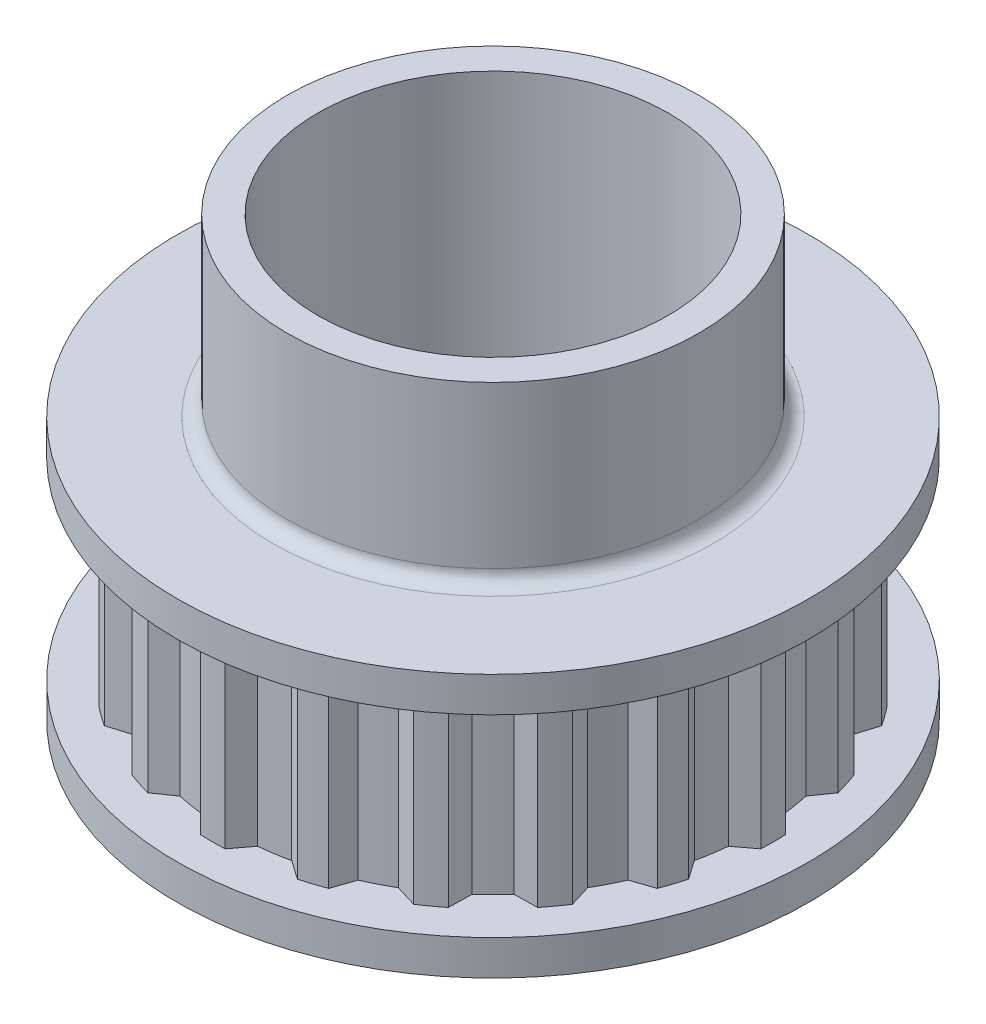
SolidWorks part; units mm, degrees
ref_plane "Front Plane" through (0, 0, 0) normal (0, 0, 1) x (1, 0, 0)
ref_plane "Top Plane" through (0, 0, 0) normal (0, 1, 0) x (1, 0, 0)
ref_plane "Right Plane" through (0, 0, 0) normal (1, 0, 0) x (0, 0, -1)
sketch "Sketch1" plane through (0, 0, 0) normal (0, 1, 0) x (1, 0, 0)
  circle A0 centre (0, 0) radius 16
  dimension "D1" = 32
extrude "Boss-Extrude1" add sketch "Sketch1" along normal blind 11
sketch "Sketch2" plane through (0, 11, 0) normal (0, 1, 0) x (1, 0, 0)
  line L0 (0, 21.2272) -> (0, -27.4763) construction
  line L1 (-1.5, 14.9329) -> (-0.7089, 15.9843)
  line L2 (1.5, 14.9329) -> (0.7089, 15.9843)
  line L3 (3.1879, 14.6656) -> (4.2652, 15.421)
  line L4 (6.0411, 13.7385) -> (5.6137, 14.9829)
  line L5 (7.5638, 12.9627) -> (8.8218, 13.3483)
  line L6 (9.9909, 11.1993) -> (9.9689, 12.5149)
  line L7 (11.1993, 9.9909) -> (12.5149, 9.9689)
  line L8 (12.9627, 7.5638) -> (13.3483, 8.8218)
  line L9 (13.7385, 6.0411) -> (14.9829, 5.6137)
  line L10 (14.6656, 3.1879) -> (15.421, 4.2652)
  line L11 (14.9329, 1.5) -> (15.9843, 0.7089)
  line L12 (14.9329, -1.5) -> (15.9843, -0.7089)
  line L13 (14.6656, -3.1879) -> (15.421, -4.2652)
  line L14 (13.7385, -6.0411) -> (14.9829, -5.6137)
  line L15 (12.9627, -7.5638) -> (13.3483, -8.8218)
  line L16 (11.1993, -9.9909) -> (12.5149, -9.9689)
  line L17 (9.9909, -11.1993) -> (9.9689, -12.5149)
  line L18 (7.5638, -12.9627) -> (8.8218, -13.3483)
  line L19 (6.0411, -13.7385) -> (5.6137, -14.9829)
  line L20 (3.1879, -14.6656) -> (4.2652, -15.421)
  line L21 (1.5, -14.9329) -> (0.7089, -15.9843)
  line L22 (-1.5, -14.9329) -> (-0.7089, -15.9843)
  line L23 (-3.1879, -14.6656) -> (-4.2652, -15.421)
  line L24 (-6.0411, -13.7385) -> (-5.6137, -14.9829)
  line L25 (-7.5638, -12.9627) -> (-8.8218, -13.3483)
  line L26 (-9.9909, -11.1993) -> (-9.9689, -12.5149)
  line L27 (-11.1993, -9.9909) -> (-12.5149, -9.9689)
  line L28 (-12.9627, -7.5638) -> (-13.3483, -8.8218)
  line L29 (-13.7385, -6.0411) -> (-14.9829, -5.6137)
  line L30 (-14.6656, -3.1879) -> (-15.421, -4.2652)
  line L31 (-14.9329, -1.5) -> (-15.9843, -0.7089)
  line L32 (-14.9329, 1.5) -> (-15.9843, 0.7089)
  line L33 (-14.6656, 3.1879) -> (-15.421, 4.2652)
  line L34 (-13.7385, 6.0411) -> (-14.9829, 5.6137)
  line L35 (-12.9627, 7.5638) -> (-13.3483, 8.8218)
  line L36 (-11.1993, 9.9909) -> (-12.5149, 9.9689)
  line L37 (-9.9909, 11.1993) -> (-9.9689, 12.5149)
  line L38 (-7.5638, 12.9627) -> (-8.8218, 13.3483)
  line L39 (-6.0411, 13.7385) -> (-5.6137, 14.9829)
  line L40 (-3.1879, 14.6656) -> (-4.2652, 15.421)
  arc A0 (-1.5, 14.9329) -> (-3.1879, 14.6656) centre (0, 0) ccw
  circle A1 centre (0, 0) radius 16 construction
  arc A3 (-1.5, 14.9329) -> (-3.1879, 14.6656) centre (0, 0) ccw
  arc A4 (5.6137, 14.9829) -> (4.2652, 15.421) centre (0, 0) ccw
  arc A5 (-1.5, 14.9329) -> (-3.1879, 14.6656) centre (0, 0) ccw
  arc A6 (9.9689, 12.5149) -> (8.8218, 13.3483) centre (0, 0) ccw
  arc A7 (-1.5, 14.9329) -> (-3.1879, 14.6656) centre (0, 0) ccw
  arc A8 (13.3483, 8.8218) -> (12.5149, 9.9689) centre (0, 0) ccw
  arc A9 (-1.5, 14.9329) -> (-3.1879, 14.6656) centre (0, 0) ccw
  arc A10 (15.9843, 0.7089) -> (15.421, 4.2652) centre (0, 0) ccw
  arc A11 (-1.5, 14.9329) -> (-3.1879, 14.6656) centre (0, 0) ccw
  arc A12 (15.421, -4.2652) -> (15.9843, -0.7089) centre (0, 0) ccw
  arc A13 (-1.5, 14.9329) -> (-3.1879, 14.6656) centre (0, 0) ccw
  arc A14 (13.3483, -8.8218) -> (14.9829, -5.6137) centre (0, 0) ccw
  arc A15 (-1.5, 14.9329) -> (-3.1879, 14.6656) centre (0, 0) ccw
  arc A16 (9.9689, -12.5149) -> (12.5149, -9.9689) centre (0, 0) ccw
  arc A17 (-1.5, 14.9329) -> (-3.1879, 14.6656) centre (0, 0) ccw
  arc A18 (5.6137, -14.9829) -> (8.8218, -13.3483) centre (0, 0) ccw
  arc A19 (-1.5, 14.9329) -> (-3.1879, 14.6656) centre (0, 0) ccw
  arc A20 (0.7089, -15.9843) -> (4.2652, -15.421) centre (0, 0) ccw
  arc A21 (-1.5, 14.9329) -> (-3.1879, 14.6656) centre (0, 0) ccw
  arc A22 (-4.2652, -15.421) -> (-0.7089, -15.9843) centre (0, 0) ccw
  arc A23 (-1.5, 14.9329) -> (-3.1879, 14.6656) centre (0, 0) ccw
  arc A24 (-8.8218, -13.3483) -> (-5.6137, -14.9829) centre (0, 0) ccw
  arc A25 (-1.5, 14.9329) -> (-3.1879, 14.6656) centre (0, 0) ccw
  arc A26 (-12.5149, -9.9689) -> (-9.9689, -12.5149) centre (0, 0) ccw
  arc A27 (-1.5, 14.9329) -> (-3.1879, 14.6656) centre (0, 0) ccw
  arc A28 (-14.9829, -5.6137) -> (-13.3483, -8.8218) centre (0, 0) ccw
  arc A29 (-1.5, 14.9329) -> (-3.1879, 14.6656) centre (0, 0) ccw
  arc A30 (-15.9843, -0.7089) -> (-15.421, -4.2652) centre (0, 0) ccw
  arc A31 (-1.5, 14.9329) -> (-3.1879, 14.6656) centre (0, 0) ccw
  arc A32 (-15.421, 4.2652) -> (-15.9843, 0.7089) centre (0, 0) ccw
  arc A33 (-1.5, 14.9329) -> (-3.1879, 14.6656) centre (0, 0) ccw
  arc A34 (-13.3483, 8.8218) -> (-14.9829, 5.6137) centre (0, 0) ccw
  arc A35 (-1.5, 14.9329) -> (-3.1879, 14.6656) centre (0, 0) ccw
  arc A36 (-9.9689, 12.5149) -> (-12.5149, 9.9689) centre (0, 0) ccw
  arc A37 (-1.5, 14.9329) -> (-3.1879, 14.6656) centre (0, 0) ccw
  arc A38 (-5.6137, 14.9829) -> (-8.8218, 13.3483) centre (0, 0) ccw
  arc A39 (-1.5, 14.9329) -> (-3.1879, 14.6656) centre (0, 0) ccw
  arc A40 (-0.7089, 15.9843) -> (-4.2652, 15.421) centre (0, 0) ccw
  arc A41 (3.1879, 14.6656) -> (1.5, 14.9329) centre (0, 0) ccw
  arc A42 (3.1879, 14.6656) -> (1.5, 14.9329) centre (0, 0) ccw
  arc A43 (3.1879, 14.6656) -> (1.5, 14.9329) centre (0, 0) ccw
  arc A44 (3.1879, 14.6656) -> (1.5, 14.9329) centre (0, 0) ccw
  arc A45 (3.1879, 14.6656) -> (1.5, 14.9329) centre (0, 0) ccw
  arc A46 (3.1879, 14.6656) -> (1.5, 14.9329) centre (0, 0) ccw
  arc A47 (3.1879, 14.6656) -> (1.5, 14.9329) centre (0, 0) ccw
  arc A48 (3.1879, 14.6656) -> (1.5, 14.9329) centre (0, 0) ccw
  arc A49 (3.1879, 14.6656) -> (1.5, 14.9329) centre (0, 0) ccw
  arc A50 (3.1879, 14.6656) -> (1.5, 14.9329) centre (0, 0) ccw
  arc A51 (3.1879, 14.6656) -> (1.5, 14.9329) centre (0, 0) ccw
  arc A52 (3.1879, 14.6656) -> (1.5, 14.9329) centre (0, 0) ccw
  arc A53 (3.1879, 14.6656) -> (1.5, 14.9329) centre (0, 0) ccw
  arc A54 (3.1879, 14.6656) -> (1.5, 14.9329) centre (0, 0) ccw
  arc A55 (3.1879, 14.6656) -> (1.5, 14.9329) centre (0, 0) ccw
  arc A56 (3.1879, 14.6656) -> (1.5, 14.9329) centre (0, 0) ccw
  arc A57 (3.1879, 14.6656) -> (1.5, 14.9329) centre (0, 0) ccw
  arc A58 (3.1879, 14.6656) -> (1.5, 14.9329) centre (0, 0) ccw
  arc A59 (3.1879, 14.6656) -> (1.5, 14.9329) centre (0, 0) ccw
  arc A60 (3.1879, 14.6656) -> (1.5, 14.9329) centre (0, 0) ccw
  arc A61 (7.5638, 12.9627) -> (6.0411, 13.7385) centre (0, 0) ccw
  arc A62 (7.5638, 12.9627) -> (6.0411, 13.7385) centre (0, 0) ccw
  arc A63 (7.5638, 12.9627) -> (6.0411, 13.7385) centre (0, 0) ccw
  arc A64 (7.5638, 12.9627) -> (6.0411, 13.7385) centre (0, 0) ccw
  arc A65 (7.5638, 12.9627) -> (6.0411, 13.7385) centre (0, 0) ccw
  arc A66 (7.5638, 12.9627) -> (6.0411, 13.7385) centre (0, 0) ccw
  arc A67 (7.5638, 12.9627) -> (6.0411, 13.7385) centre (0, 0) ccw
  arc A68 (7.5638, 12.9627) -> (6.0411, 13.7385) centre (0, 0) ccw
  arc A69 (7.5638, 12.9627) -> (6.0411, 13.7385) centre (0, 0) ccw
  arc A70 (7.5638, 12.9627) -> (6.0411, 13.7385) centre (0, 0) ccw
  arc A71 (7.5638, 12.9627) -> (6.0411, 13.7385) centre (0, 0) ccw
  arc A72 (7.5638, 12.9627) -> (6.0411, 13.7385) centre (0, 0) ccw
  arc A73 (7.5638, 12.9627) -> (6.0411, 13.7385) centre (0, 0) ccw
  arc A74 (7.5638, 12.9627) -> (6.0411, 13.7385) centre (0, 0) ccw
  arc A75 (7.5638, 12.9627) -> (6.0411, 13.7385) centre (0, 0) ccw
  arc A76 (7.5638, 12.9627) -> (6.0411, 13.7385) centre (0, 0) ccw
  arc A77 (7.5638, 12.9627) -> (6.0411, 13.7385) centre (0, 0) ccw
  arc A78 (7.5638, 12.9627) -> (6.0411, 13.7385) centre (0, 0) ccw
  arc A79 (7.5638, 12.9627) -> (6.0411, 13.7385) centre (0, 0) ccw
  arc A80 (7.5638, 12.9627) -> (6.0411, 13.7385) centre (0, 0) ccw
  arc A81 (11.1993, 9.9909) -> (9.9909, 11.1993) centre (0, 0) ccw
  arc A82 (11.1993, 9.9909) -> (9.9909, 11.1993) centre (0, 0) ccw
  arc A83 (11.1993, 9.9909) -> (9.9909, 11.1993) centre (0, 0) ccw
  arc A84 (11.1993, 9.9909) -> (9.9909, 11.1993) centre (0, 0) ccw
  arc A85 (11.1993, 9.9909) -> (9.9909, 11.1993) centre (0, 0) ccw
  arc A86 (11.1993, 9.9909) -> (9.9909, 11.1993) centre (0, 0) ccw
  arc A87 (11.1993, 9.9909) -> (9.9909, 11.1993) centre (0, 0) ccw
  arc A88 (11.1993, 9.9909) -> (9.9909, 11.1993) centre (0, 0) ccw
  arc A89 (11.1993, 9.9909) -> (9.9909, 11.1993) centre (0, 0) ccw
  arc A90 (11.1993, 9.9909) -> (9.9909, 11.1993) centre (0, 0) ccw
  arc A91 (11.1993, 9.9909) -> (9.9909, 11.1993) centre (0, 0) ccw
  arc A92 (11.1993, 9.9909) -> (9.9909, 11.1993) centre (0, 0) ccw
  arc A93 (11.1993, 9.9909) -> (9.9909, 11.1993) centre (0, 0) ccw
  arc A94 (11.1993, 9.9909) -> (9.9909, 11.1993) centre (0, 0) ccw
  arc A95 (11.1993, 9.9909) -> (9.9909, 11.1993) centre (0, 0) ccw
  arc A96 (11.1993, 9.9909) -> (9.9909, 11.1993) centre (0, 0) ccw
  arc A97 (11.1993, 9.9909) -> (9.9909, 11.1993) centre (0, 0) ccw
  arc A98 (11.1993, 9.9909) -> (9.9909, 11.1993) centre (0, 0) ccw
  arc A99 (11.1993, 9.9909) -> (9.9909, 11.1993) centre (0, 0) ccw
  arc A100 (11.1993, 9.9909) -> (9.9909, 11.1993) centre (0, 0) ccw
  arc A101 (13.7385, 6.0411) -> (12.9627, 7.5638) centre (0, 0) ccw
  arc A102 (13.7385, 6.0411) -> (12.9627, 7.5638) centre (0, 0) ccw
  arc A103 (13.7385, 6.0411) -> (12.9627, 7.5638) centre (0, 0) ccw
  arc A104 (13.7385, 6.0411) -> (12.9627, 7.5638) centre (0, 0) ccw
  arc A105 (13.7385, 6.0411) -> (12.9627, 7.5638) centre (0, 0) ccw
  arc A106 (13.7385, 6.0411) -> (12.9627, 7.5638) centre (0, 0) ccw
  arc A107 (13.7385, 6.0411) -> (12.9627, 7.5638) centre (0, 0) ccw
  arc A108 (13.7385, 6.0411) -> (12.9627, 7.5638) centre (0, 0) ccw
  arc A109 (13.7385, 6.0411) -> (12.9627, 7.5638) centre (0, 0) ccw
  arc A110 (13.7385, 6.0411) -> (12.9627, 7.5638) centre (0, 0) ccw
  arc A111 (13.7385, 6.0411) -> (12.9627, 7.5638) centre (0, 0) ccw
  arc A112 (13.7385, 6.0411) -> (12.9627, 7.5638) centre (0, 0) ccw
  arc A113 (13.7385, 6.0411) -> (12.9627, 7.5638) centre (0, 0) ccw
  arc A114 (13.7385, 6.0411) -> (12.9627, 7.5638) centre (0, 0) ccw
  arc A115 (13.7385, 6.0411) -> (12.9627, 7.5638) centre (0, 0) ccw
  arc A116 (13.7385, 6.0411) -> (12.9627, 7.5638) centre (0, 0) ccw
  arc A117 (13.7385, 6.0411) -> (12.9627, 7.5638) centre (0, 0) ccw
  arc A118 (13.7385, 6.0411) -> (12.9627, 7.5638) centre (0, 0) ccw
  arc A119 (13.7385, 6.0411) -> (12.9627, 7.5638) centre (0, 0) ccw
  arc A120 (13.7385, 6.0411) -> (12.9627, 7.5638) centre (0, 0) ccw
  arc A121 (14.9329, 1.5) -> (14.6656, 3.1879) centre (0, 0) ccw
  arc A122 (14.9329, 1.5) -> (14.6656, 3.1879) centre (0, 0) ccw
  arc A123 (14.9329, 1.5) -> (14.6656, 3.1879) centre (0, 0) ccw
  arc A124 (14.9329, 1.5) -> (14.6656, 3.1879) centre (0, 0) ccw
  arc A125 (14.9329, 1.5) -> (14.6656, 3.1879) centre (0, 0) ccw
  arc A126 (14.9329, 1.5) -> (14.6656, 3.1879) centre (0, 0) ccw
  arc A127 (14.9329, 1.5) -> (14.6656, 3.1879) centre (0, 0) ccw
  arc A128 (14.9329, 1.5) -> (14.6656, 3.1879) centre (0, 0) ccw
  arc A129 (14.9329, 1.5) -> (14.6656, 3.1879) centre (0, 0) ccw
  arc A130 (14.9329, 1.5) -> (14.6656, 3.1879) centre (0, 0) ccw
  arc A131 (14.9329, 1.5) -> (14.6656, 3.1879) centre (0, 0) ccw
  arc A132 (14.9329, 1.5) -> (14.6656, 3.1879) centre (0, 0) ccw
  arc A133 (14.9329, 1.5) -> (14.6656, 3.1879) centre (0, 0) ccw
  arc A134 (14.9329, 1.5) -> (14.6656, 3.1879) centre (0, 0) ccw
  arc A135 (14.9329, 1.5) -> (14.6656, 3.1879) centre (0, 0) ccw
  arc A136 (14.9329, 1.5) -> (14.6656, 3.1879) centre (0, 0) ccw
  arc A137 (14.9329, 1.5) -> (14.6656, 3.1879) centre (0, 0) ccw
  arc A138 (14.9329, 1.5) -> (14.6656, 3.1879) centre (0, 0) ccw
  arc A139 (14.9329, 1.5) -> (14.6656, 3.1879) centre (0, 0) ccw
  arc A140 (14.9329, 1.5) -> (14.6656, 3.1879) centre (0, 0) ccw
  arc A141 (14.6656, -3.1879) -> (14.9329, -1.5) centre (0, 0) ccw
  arc A142 (14.6656, -3.1879) -> (14.9329, -1.5) centre (0, 0) ccw
  arc A143 (14.6656, -3.1879) -> (14.9329, -1.5) centre (0, 0) ccw
  arc A144 (14.6656, -3.1879) -> (14.9329, -1.5) centre (0, 0) ccw
  arc A145 (14.6656, -3.1879) -> (14.9329, -1.5) centre (0, 0) ccw
  arc A146 (14.6656, -3.1879) -> (14.9329, -1.5) centre (0, 0) ccw
  arc A147 (14.6656, -3.1879) -> (14.9329, -1.5) centre (0, 0) ccw
  arc A148 (14.6656, -3.1879) -> (14.9329, -1.5) centre (0, 0) ccw
  arc A149 (14.6656, -3.1879) -> (14.9329, -1.5) centre (0, 0) ccw
  arc A150 (14.6656, -3.1879) -> (14.9329, -1.5) centre (0, 0) ccw
  arc A151 (14.6656, -3.1879) -> (14.9329, -1.5) centre (0, 0) ccw
  arc A152 (14.6656, -3.1879) -> (14.9329, -1.5) centre (0, 0) ccw
  arc A153 (14.6656, -3.1879) -> (14.9329, -1.5) centre (0, 0) ccw
  arc A154 (14.6656, -3.1879) -> (14.9329, -1.5) centre (0, 0) ccw
  arc A155 (14.6656, -3.1879) -> (14.9329, -1.5) centre (0, 0) ccw
  arc A156 (14.6656, -3.1879) -> (14.9329, -1.5) centre (0, 0) ccw
  arc A157 (14.6656, -3.1879) -> (14.9329, -1.5) centre (0, 0) ccw
  arc A158 (14.6656, -3.1879) -> (14.9329, -1.5) centre (0, 0) ccw
  arc A159 (14.6656, -3.1879) -> (14.9329, -1.5) centre (0, 0) ccw
  arc A160 (14.6656, -3.1879) -> (14.9329, -1.5) centre (0, 0) ccw
  arc A161 (12.9627, -7.5638) -> (13.7385, -6.0411) centre (0, 0) ccw
  arc A162 (12.9627, -7.5638) -> (13.7385, -6.0411) centre (0, 0) ccw
  arc A163 (12.9627, -7.5638) -> (13.7385, -6.0411) centre (0, 0) ccw
  arc A164 (12.9627, -7.5638) -> (13.7385, -6.0411) centre (0, 0) ccw
  arc A165 (12.9627, -7.5638) -> (13.7385, -6.0411) centre (0, 0) ccw
  arc A166 (12.9627, -7.5638) -> (13.7385, -6.0411) centre (0, 0) ccw
  arc A167 (12.9627, -7.5638) -> (13.7385, -6.0411) centre (0, 0) ccw
  arc A168 (12.9627, -7.5638) -> (13.7385, -6.0411) centre (0, 0) ccw
  arc A169 (12.9627, -7.5638) -> (13.7385, -6.0411) centre (0, 0) ccw
  arc A170 (12.9627, -7.5638) -> (13.7385, -6.0411) centre (0, 0) ccw
  arc A171 (12.9627, -7.5638) -> (13.7385, -6.0411) centre (0, 0) ccw
  arc A172 (12.9627, -7.5638) -> (13.7385, -6.0411) centre (0, 0) ccw
  arc A173 (12.9627, -7.5638) -> (13.7385, -6.0411) centre (0, 0) ccw
  arc A174 (12.9627, -7.5638) -> (13.7385, -6.0411) centre (0, 0) ccw
  arc A175 (12.9627, -7.5638) -> (13.7385, -6.0411) centre (0, 0) ccw
  arc A176 (12.9627, -7.5638) -> (13.7385, -6.0411) centre (0, 0) ccw
  arc A177 (12.9627, -7.5638) -> (13.7385, -6.0411) centre (0, 0) ccw
  arc A178 (12.9627, -7.5638) -> (13.7385, -6.0411) centre (0, 0) ccw
  arc A179 (12.9627, -7.5638) -> (13.7385, -6.0411) centre (0, 0) ccw
  arc A180 (12.9627, -7.5638) -> (13.7385, -6.0411) centre (0, 0) ccw
  arc A181 (9.9909, -11.1993) -> (11.1993, -9.9909) centre (0, 0) ccw
  arc A182 (9.9909, -11.1993) -> (11.1993, -9.9909) centre (0, 0) ccw
  arc A183 (9.9909, -11.1993) -> (11.1993, -9.9909) centre (0, 0) ccw
  arc A184 (9.9909, -11.1993) -> (11.1993, -9.9909) centre (0, 0) ccw
  arc A185 (9.9909, -11.1993) -> (11.1993, -9.9909) centre (0, 0) ccw
  arc A186 (9.9909, -11.1993) -> (11.1993, -9.9909) centre (0, 0) ccw
  arc A187 (9.9909, -11.1993) -> (11.1993, -9.9909) centre (0, 0) ccw
  arc A188 (9.9909, -11.1993) -> (11.1993, -9.9909) centre (0, 0) ccw
  arc A189 (9.9909, -11.1993) -> (11.1993, -9.9909) centre (0, 0) ccw
  arc A190 (9.9909, -11.1993) -> (11.1993, -9.9909) centre (0, 0) ccw
  arc A191 (9.9909, -11.1993) -> (11.1993, -9.9909) centre (0, 0) ccw
  arc A192 (9.9909, -11.1993) -> (11.1993, -9.9909) centre (0, 0) ccw
  arc A193 (9.9909, -11.1993) -> (11.1993, -9.9909) centre (0, 0) ccw
  arc A194 (9.9909, -11.1993) -> (11.1993, -9.9909) centre (0, 0) ccw
  arc A195 (9.9909, -11.1993) -> (11.1993, -9.9909) centre (0, 0) ccw
  arc A196 (9.9909, -11.1993) -> (11.1993, -9.9909) centre (0, 0) ccw
  arc A197 (9.9909, -11.1993) -> (11.1993, -9.9909) centre (0, 0) ccw
  arc A198 (9.9909, -11.1993) -> (11.1993, -9.9909) centre (0, 0) ccw
  arc A199 (9.9909, -11.1993) -> (11.1993, -9.9909) centre (0, 0) ccw
  arc A200 (9.9909, -11.1993) -> (11.1993, -9.9909) centre (0, 0) ccw
  arc A201 (1.5, -14.9329) -> (3.1879, -14.6656) centre (0, 0) ccw
  arc A202 (1.5, -14.9329) -> (3.1879, -14.6656) centre (0, 0) ccw
  arc A203 (1.5, -14.9329) -> (3.1879, -14.6656) centre (0, 0) ccw
  arc A204 (1.5, -14.9329) -> (3.1879, -14.6656) centre (0, 0) ccw
  arc A205 (1.5, -14.9329) -> (3.1879, -14.6656) centre (0, 0) ccw
  arc A206 (1.5, -14.9329) -> (3.1879, -14.6656) centre (0, 0) ccw
  arc A207 (1.5, -14.9329) -> (3.1879, -14.6656) centre (0, 0) ccw
  arc A208 (1.5, -14.9329) -> (3.1879, -14.6656) centre (0, 0) ccw
  arc A209 (1.5, -14.9329) -> (3.1879, -14.6656) centre (0, 0) ccw
  arc A210 (1.5, -14.9329) -> (3.1879, -14.6656) centre (0, 0) ccw
  arc A211 (1.5, -14.9329) -> (3.1879, -14.6656) centre (0, 0) ccw
  arc A212 (1.5, -14.9329) -> (3.1879, -14.6656) centre (0, 0) ccw
  arc A213 (1.5, -14.9329) -> (3.1879, -14.6656) centre (0, 0) ccw
  arc A214 (1.5, -14.9329) -> (3.1879, -14.6656) centre (0, 0) ccw
  arc A215 (1.5, -14.9329) -> (3.1879, -14.6656) centre (0, 0) ccw
  arc A216 (1.5, -14.9329) -> (3.1879, -14.6656) centre (0, 0) ccw
  arc A217 (1.5, -14.9329) -> (3.1879, -14.6656) centre (0, 0) ccw
  arc A218 (1.5, -14.9329) -> (3.1879, -14.6656) centre (0, 0) ccw
  arc A219 (1.5, -14.9329) -> (3.1879, -14.6656) centre (0, 0) ccw
  arc A220 (1.5, -14.9329) -> (3.1879, -14.6656) centre (0, 0) ccw
  arc A221 (-3.1879, -14.6656) -> (-1.5, -14.9329) centre (0, 0) ccw
  arc A222 (-3.1879, -14.6656) -> (-1.5, -14.9329) centre (0, 0) ccw
  arc A223 (-3.1879, -14.6656) -> (-1.5, -14.9329) centre (0, 0) ccw
  arc A224 (-3.1879, -14.6656) -> (-1.5, -14.9329) centre (0, 0) ccw
  arc A225 (-3.1879, -14.6656) -> (-1.5, -14.9329) centre (0, 0) ccw
  arc A226 (-3.1879, -14.6656) -> (-1.5, -14.9329) centre (0, 0) ccw
  arc A227 (-3.1879, -14.6656) -> (-1.5, -14.9329) centre (0, 0) ccw
  arc A228 (-3.1879, -14.6656) -> (-1.5, -14.9329) centre (0, 0) ccw
  arc A229 (-3.1879, -14.6656) -> (-1.5, -14.9329) centre (0, 0) ccw
  arc A230 (-3.1879, -14.6656) -> (-1.5, -14.9329) centre (0, 0) ccw
  arc A231 (-3.1879, -14.6656) -> (-1.5, -14.9329) centre (0, 0) ccw
  arc A232 (-3.1879, -14.6656) -> (-1.5, -14.9329) centre (0, 0) ccw
  arc A233 (-3.1879, -14.6656) -> (-1.5, -14.9329) centre (0, 0) ccw
  arc A234 (-3.1879, -14.6656) -> (-1.5, -14.9329) centre (0, 0) ccw
  arc A235 (-3.1879, -14.6656) -> (-1.5, -14.9329) centre (0, 0) ccw
  arc A236 (-3.1879, -14.6656) -> (-1.5, -14.9329) centre (0, 0) ccw
  arc A237 (-3.1879, -14.6656) -> (-1.5, -14.9329) centre (0, 0) ccw
  arc A238 (-3.1879, -14.6656) -> (-1.5, -14.9329) centre (0, 0) ccw
  arc A239 (-3.1879, -14.6656) -> (-1.5, -14.9329) centre (0, 0) ccw
  arc A240 (-3.1879, -14.6656) -> (-1.5, -14.9329) centre (0, 0) ccw
  arc A241 (-7.5638, -12.9627) -> (-6.0411, -13.7385) centre (0, 0) ccw
  arc A242 (-7.5638, -12.9627) -> (-6.0411, -13.7385) centre (0, 0) ccw
  arc A243 (-7.5638, -12.9627) -> (-6.0411, -13.7385) centre (0, 0) ccw
  arc A244 (-7.5638, -12.9627) -> (-6.0411, -13.7385) centre (0, 0) ccw
  arc A245 (-7.5638, -12.9627) -> (-6.0411, -13.7385) centre (0, 0) ccw
  arc A246 (-7.5638, -12.9627) -> (-6.0411, -13.7385) centre (0, 0) ccw
  arc A247 (-7.5638, -12.9627) -> (-6.0411, -13.7385) centre (0, 0) ccw
  arc A248 (-7.5638, -12.9627) -> (-6.0411, -13.7385) centre (0, 0) ccw
  arc A249 (-7.5638, -12.9627) -> (-6.0411, -13.7385) centre (0, 0) ccw
  arc A250 (-7.5638, -12.9627) -> (-6.0411, -13.7385) centre (0, 0) ccw
  arc A251 (-7.5638, -12.9627) -> (-6.0411, -13.7385) centre (0, 0) ccw
  arc A252 (-7.5638, -12.9627) -> (-6.0411, -13.7385) centre (0, 0) ccw
  arc A253 (-7.5638, -12.9627) -> (-6.0411, -13.7385) centre (0, 0) ccw
  arc A254 (-7.5638, -12.9627) -> (-6.0411, -13.7385) centre (0, 0) ccw
  arc A255 (-7.5638, -12.9627) -> (-6.0411, -13.7385) centre (0, 0) ccw
  arc A256 (-7.5638, -12.9627) -> (-6.0411, -13.7385) centre (0, 0) ccw
  arc A257 (-7.5638, -12.9627) -> (-6.0411, -13.7385) centre (0, 0) ccw
  arc A258 (-7.5638, -12.9627) -> (-6.0411, -13.7385) centre (0, 0) ccw
  arc A259 (-7.5638, -12.9627) -> (-6.0411, -13.7385) centre (0, 0) ccw
  arc A260 (-7.5638, -12.9627) -> (-6.0411, -13.7385) centre (0, 0) ccw
  arc A261 (-11.1993, -9.9909) -> (-9.9909, -11.1993) centre (0, 0) ccw
  arc A262 (-11.1993, -9.9909) -> (-9.9909, -11.1993) centre (0, 0) ccw
  arc A263 (-11.1993, -9.9909) -> (-9.9909, -11.1993) centre (0, 0) ccw
  arc A264 (-11.1993, -9.9909) -> (-9.9909, -11.1993) centre (0, 0) ccw
  arc A265 (-11.1993, -9.9909) -> (-9.9909, -11.1993) centre (0, 0) ccw
  arc A266 (-11.1993, -9.9909) -> (-9.9909, -11.1993) centre (0, 0) ccw
  arc A267 (-11.1993, -9.9909) -> (-9.9909, -11.1993) centre (0, 0) ccw
  arc A268 (-11.1993, -9.9909) -> (-9.9909, -11.1993) centre (0, 0) ccw
  arc A269 (-11.1993, -9.9909) -> (-9.9909, -11.1993) centre (0, 0) ccw
  arc A270 (-11.1993, -9.9909) -> (-9.9909, -11.1993) centre (0, 0) ccw
  arc A271 (-11.1993, -9.9909) -> (-9.9909, -11.1993) centre (0, 0) ccw
  arc A272 (-11.1993, -9.9909) -> (-9.9909, -11.1993) centre (0, 0) ccw
  arc A273 (-11.1993, -9.9909) -> (-9.9909, -11.1993) centre (0, 0) ccw
  arc A274 (-11.1993, -9.9909) -> (-9.9909, -11.1993) centre (0, 0) ccw
  arc A275 (-11.1993, -9.9909) -> (-9.9909, -11.1993) centre (0, 0) ccw
  arc A276 (-11.1993, -9.9909) -> (-9.9909, -11.1993) centre (0, 0) ccw
  arc A277 (-11.1993, -9.9909) -> (-9.9909, -11.1993) centre (0, 0) ccw
  arc A278 (-11.1993, -9.9909) -> (-9.9909, -11.1993) centre (0, 0) ccw
  arc A279 (-11.1993, -9.9909) -> (-9.9909, -11.1993) centre (0, 0) ccw
  arc A280 (-11.1993, -9.9909) -> (-9.9909, -11.1993) centre (0, 0) ccw
  arc A281 (-13.7385, -6.0411) -> (-12.9627, -7.5638) centre (0, 0) ccw
  arc A282 (-13.7385, -6.0411) -> (-12.9627, -7.5638) centre (0, 0) ccw
  arc A283 (-13.7385, -6.0411) -> (-12.9627, -7.5638) centre (0, 0) ccw
  arc A284 (-13.7385, -6.0411) -> (-12.9627, -7.5638) centre (0, 0) ccw
  arc A285 (-13.7385, -6.0411) -> (-12.9627, -7.5638) centre (0, 0) ccw
  arc A286 (-13.7385, -6.0411) -> (-12.9627, -7.5638) centre (0, 0) ccw
  arc A287 (-13.7385, -6.0411) -> (-12.9627, -7.5638) centre (0, 0) ccw
  arc A288 (-13.7385, -6.0411) -> (-12.9627, -7.5638) centre (0, 0) ccw
  arc A289 (-13.7385, -6.0411) -> (-12.9627, -7.5638) centre (0, 0) ccw
  arc A290 (-13.7385, -6.0411) -> (-12.9627, -7.5638) centre (0, 0) ccw
  arc A291 (-13.7385, -6.0411) -> (-12.9627, -7.5638) centre (0, 0) ccw
  arc A292 (-13.7385, -6.0411) -> (-12.9627, -7.5638) centre (0, 0) ccw
  arc A293 (-13.7385, -6.0411) -> (-12.9627, -7.5638) centre (0, 0) ccw
  arc A294 (-13.7385, -6.0411) -> (-12.9627, -7.5638) centre (0, 0) ccw
  arc A295 (-13.7385, -6.0411) -> (-12.9627, -7.5638) centre (0, 0) ccw
  arc A296 (-13.7385, -6.0411) -> (-12.9627, -7.5638) centre (0, 0) ccw
  arc A297 (-13.7385, -6.0411) -> (-12.9627, -7.5638) centre (0, 0) ccw
  arc A298 (-13.7385, -6.0411) -> (-12.9627, -7.5638) centre (0, 0) ccw
  arc A299 (-13.7385, -6.0411) -> (-12.9627, -7.5638) centre (0, 0) ccw
  arc A300 (-13.7385, -6.0411) -> (-12.9627, -7.5638) centre (0, 0) ccw
  arc A301 (-14.9329, -1.5) -> (-14.6656, -3.1879) centre (0, 0) ccw
  arc A302 (-14.9329, -1.5) -> (-14.6656, -3.1879) centre (0, 0) ccw
  arc A303 (-14.9329, -1.5) -> (-14.6656, -3.1879) centre (0, 0) ccw
  arc A304 (-14.9329, -1.5) -> (-14.6656, -3.1879) centre (0, 0) ccw
  arc A305 (-14.9329, -1.5) -> (-14.6656, -3.1879) centre (0, 0) ccw
  arc A306 (-14.9329, -1.5) -> (-14.6656, -3.1879) centre (0, 0) ccw
  arc A307 (-14.9329, -1.5) -> (-14.6656, -3.1879) centre (0, 0) ccw
  arc A308 (-14.9329, -1.5) -> (-14.6656, -3.1879) centre (0, 0) ccw
  arc A309 (-14.9329, -1.5) -> (-14.6656, -3.1879) centre (0, 0) ccw
  arc A310 (-14.9329, -1.5) -> (-14.6656, -3.1879) centre (0, 0) ccw
  arc A311 (-14.9329, -1.5) -> (-14.6656, -3.1879) centre (0, 0) ccw
  arc A312 (-14.9329, -1.5) -> (-14.6656, -3.1879) centre (0, 0) ccw
  arc A313 (-14.9329, -1.5) -> (-14.6656, -3.1879) centre (0, 0) ccw
  arc A314 (-14.9329, -1.5) -> (-14.6656, -3.1879) centre (0, 0) ccw
  arc A315 (-14.9329, -1.5) -> (-14.6656, -3.1879) centre (0, 0) ccw
  arc A316 (-14.9329, -1.5) -> (-14.6656, -3.1879) centre (0, 0) ccw
  arc A317 (-14.9329, -1.5) -> (-14.6656, -3.1879) centre (0, 0) ccw
  arc A318 (-14.9329, -1.5) -> (-14.6656, -3.1879) centre (0, 0) ccw
  arc A319 (-14.9329, -1.5) -> (-14.6656, -3.1879) centre (0, 0) ccw
  arc A320 (-14.9329, -1.5) -> (-14.6656, -3.1879) centre (0, 0) ccw
  arc A321 (-14.6656, 3.1879) -> (-14.9329, 1.5) centre (0, 0) ccw
  arc A322 (-14.6656, 3.1879) -> (-14.9329, 1.5) centre (0, 0) ccw
  arc A323 (-14.6656, 3.1879) -> (-14.9329, 1.5) centre (0, 0) ccw
  arc A324 (-14.6656, 3.1879) -> (-14.9329, 1.5) centre (0, 0) ccw
  arc A325 (-14.6656, 3.1879) -> (-14.9329, 1.5) centre (0, 0) ccw
  arc A326 (-14.6656, 3.1879) -> (-14.9329, 1.5) centre (0, 0) ccw
  arc A327 (-14.6656, 3.1879) -> (-14.9329, 1.5) centre (0, 0) ccw
  arc A328 (-14.6656, 3.1879) -> (-14.9329, 1.5) centre (0, 0) ccw
  arc A329 (-14.6656, 3.1879) -> (-14.9329, 1.5) centre (0, 0) ccw
  arc A330 (-14.6656, 3.1879) -> (-14.9329, 1.5) centre (0, 0) ccw
  arc A331 (-14.6656, 3.1879) -> (-14.9329, 1.5) centre (0, 0) ccw
  arc A332 (-14.6656, 3.1879) -> (-14.9329, 1.5) centre (0, 0) ccw
  arc A333 (-14.6656, 3.1879) -> (-14.9329, 1.5) centre (0, 0) ccw
  arc A334 (-14.6656, 3.1879) -> (-14.9329, 1.5) centre (0, 0) ccw
  arc A335 (-14.6656, 3.1879) -> (-14.9329, 1.5) centre (0, 0) ccw
  arc A336 (-14.6656, 3.1879) -> (-14.9329, 1.5) centre (0, 0) ccw
  arc A337 (-14.6656, 3.1879) -> (-14.9329, 1.5) centre (0, 0) ccw
  arc A338 (-14.6656, 3.1879) -> (-14.9329, 1.5) centre (0, 0) ccw
  arc A339 (-14.6656, 3.1879) -> (-14.9329, 1.5) centre (0, 0) ccw
  arc A340 (-14.6656, 3.1879) -> (-14.9329, 1.5) centre (0, 0) ccw
  arc A341 (-12.9627, 7.5638) -> (-13.7385, 6.0411) centre (0, 0) ccw
  arc A342 (-12.9627, 7.5638) -> (-13.7385, 6.0411) centre (0, 0) ccw
  arc A343 (-12.9627, 7.5638) -> (-13.7385, 6.0411) centre (0, 0) ccw
  arc A344 (-12.9627, 7.5638) -> (-13.7385, 6.0411) centre (0, 0) ccw
  arc A345 (-12.9627, 7.5638) -> (-13.7385, 6.0411) centre (0, 0) ccw
  arc A346 (-12.9627, 7.5638) -> (-13.7385, 6.0411) centre (0, 0) ccw
  arc A347 (-12.9627, 7.5638) -> (-13.7385, 6.0411) centre (0, 0) ccw
  arc A348 (-12.9627, 7.5638) -> (-13.7385, 6.0411) centre (0, 0) ccw
  arc A349 (-12.9627, 7.5638) -> (-13.7385, 6.0411) centre (0, 0) ccw
  arc A350 (-12.9627, 7.5638) -> (-13.7385, 6.0411) centre (0, 0) ccw
  arc A351 (-12.9627, 7.5638) -> (-13.7385, 6.0411) centre (0, 0) ccw
  arc A352 (-12.9627, 7.5638) -> (-13.7385, 6.0411) centre (0, 0) ccw
  arc A353 (-12.9627, 7.5638) -> (-13.7385, 6.0411) centre (0, 0) ccw
  arc A354 (-12.9627, 7.5638) -> (-13.7385, 6.0411) centre (0, 0) ccw
  arc A355 (-12.9627, 7.5638) -> (-13.7385, 6.0411) centre (0, 0) ccw
  arc A356 (-12.9627, 7.5638) -> (-13.7385, 6.0411) centre (0, 0) ccw
  arc A357 (-12.9627, 7.5638) -> (-13.7385, 6.0411) centre (0, 0) ccw
  arc A358 (-12.9627, 7.5638) -> (-13.7385, 6.0411) centre (0, 0) ccw
  arc A359 (-12.9627, 7.5638) -> (-13.7385, 6.0411) centre (0, 0) ccw
  arc A360 (-12.9627, 7.5638) -> (-13.7385, 6.0411) centre (0, 0) ccw
  arc A361 (-9.9909, 11.1993) -> (-11.1993, 9.9909) centre (0, 0) ccw
  arc A362 (-9.9909, 11.1993) -> (-11.1993, 9.9909) centre (0, 0) ccw
  arc A363 (-9.9909, 11.1993) -> (-11.1993, 9.9909) centre (0, 0) ccw
  arc A364 (-9.9909, 11.1993) -> (-11.1993, 9.9909) centre (0, 0) ccw
  arc A365 (-9.9909, 11.1993) -> (-11.1993, 9.9909) centre (0, 0) ccw
  arc A366 (-9.9909, 11.1993) -> (-11.1993, 9.9909) centre (0, 0) ccw
  arc A367 (-9.9909, 11.1993) -> (-11.1993, 9.9909) centre (0, 0) ccw
  arc A368 (-9.9909, 11.1993) -> (-11.1993, 9.9909) centre (0, 0) ccw
  arc A369 (-9.9909, 11.1993) -> (-11.1993, 9.9909) centre (0, 0) ccw
  arc A370 (-9.9909, 11.1993) -> (-11.1993, 9.9909) centre (0, 0) ccw
  arc A371 (-9.9909, 11.1993) -> (-11.1993, 9.9909) centre (0, 0) ccw
  arc A372 (-9.9909, 11.1993) -> (-11.1993, 9.9909) centre (0, 0) ccw
  arc A373 (-9.9909, 11.1993) -> (-11.1993, 9.9909) centre (0, 0) ccw
  arc A374 (-9.9909, 11.1993) -> (-11.1993, 9.9909) centre (0, 0) ccw
  arc A375 (-9.9909, 11.1993) -> (-11.1993, 9.9909) centre (0, 0) ccw
  arc A376 (-9.9909, 11.1993) -> (-11.1993, 9.9909) centre (0, 0) ccw
  arc A377 (-9.9909, 11.1993) -> (-11.1993, 9.9909) centre (0, 0) ccw
  arc A378 (-9.9909, 11.1993) -> (-11.1993, 9.9909) centre (0, 0) ccw
  arc A379 (-9.9909, 11.1993) -> (-11.1993, 9.9909) centre (0, 0) ccw
  arc A380 (-9.9909, 11.1993) -> (-11.1993, 9.9909) centre (0, 0) ccw
  arc A381 (-6.0411, 13.7385) -> (-7.5638, 12.9627) centre (0, 0) ccw
  arc A382 (-6.0411, 13.7385) -> (-7.5638, 12.9627) centre (0, 0) ccw
  arc A383 (-6.0411, 13.7385) -> (-7.5638, 12.9627) centre (0, 0) ccw
  arc A384 (-6.0411, 13.7385) -> (-7.5638, 12.9627) centre (0, 0) ccw
  arc A385 (-6.0411, 13.7385) -> (-7.5638, 12.9627) centre (0, 0) ccw
  arc A386 (-6.0411, 13.7385) -> (-7.5638, 12.9627) centre (0, 0) ccw
  arc A387 (-6.0411, 13.7385) -> (-7.5638, 12.9627) centre (0, 0) ccw
  arc A388 (-6.0411, 13.7385) -> (-7.5638, 12.9627) centre (0, 0) ccw
  arc A389 (-6.0411, 13.7385) -> (-7.5638, 12.9627) centre (0, 0) ccw
  arc A390 (-6.0411, 13.7385) -> (-7.5638, 12.9627) centre (0, 0) ccw
  arc A391 (-6.0411, 13.7385) -> (-7.5638, 12.9627) centre (0, 0) ccw
  arc A392 (-6.0411, 13.7385) -> (-7.5638, 12.9627) centre (0, 0) ccw
  arc A393 (-6.0411, 13.7385) -> (-7.5638, 12.9627) centre (0, 0) ccw
  arc A394 (-6.0411, 13.7385) -> (-7.5638, 12.9627) centre (0, 0) ccw
  arc A395 (-6.0411, 13.7385) -> (-7.5638, 12.9627) centre (0, 0) ccw
  arc A396 (-6.0411, 13.7385) -> (-7.5638, 12.9627) centre (0, 0) ccw
  arc A397 (-6.0411, 13.7385) -> (-7.5638, 12.9627) centre (0, 0) ccw
  arc A398 (-6.0411, 13.7385) -> (-7.5638, 12.9627) centre (0, 0) ccw
  arc A399 (-6.0411, 13.7385) -> (-7.5638, 12.9627) centre (0, 0) ccw
  arc A400 (-6.0411, 13.7385) -> (-7.5638, 12.9627) centre (0, 0) ccw
  arc A401 (14.9829, 5.6137) -> (0.7089, 15.9843) centre (0, 0) ccw
  arc A402 (6.0411, -13.7385) -> (7.5638, -12.9627) centre (0, 0) ccw
  arc A403 (6.0411, -13.7385) -> (7.5638, -12.9627) centre (0, 0) ccw
  arc A404 (6.0411, -13.7385) -> (7.5638, -12.9627) centre (0, 0) ccw
  arc A405 (6.0411, -13.7385) -> (7.5638, -12.9627) centre (0, 0) ccw
  arc A406 (6.0411, -13.7385) -> (7.5638, -12.9627) centre (0, 0) ccw
  arc A407 (6.0411, -13.7385) -> (7.5638, -12.9627) centre (0, 0) ccw
  arc A408 (6.0411, -13.7385) -> (7.5638, -12.9627) centre (0, 0) ccw
  arc A409 (6.0411, -13.7385) -> (7.5638, -12.9627) centre (0, 0) ccw
  arc A410 (6.0411, -13.7385) -> (7.5638, -12.9627) centre (0, 0) ccw
  arc A411 (6.0411, -13.7385) -> (7.5638, -12.9627) centre (0, 0) ccw
  arc A412 (6.0411, -13.7385) -> (7.5638, -12.9627) centre (0, 0) ccw
  arc A413 (6.0411, -13.7385) -> (7.5638, -12.9627) centre (0, 0) ccw
  arc A414 (6.0411, -13.7385) -> (7.5638, -12.9627) centre (0, 0) ccw
  arc A415 (6.0411, -13.7385) -> (7.5638, -12.9627) centre (0, 0) ccw
  arc A416 (6.0411, -13.7385) -> (7.5638, -12.9627) centre (0, 0) ccw
  arc A417 (6.0411, -13.7385) -> (7.5638, -12.9627) centre (0, 0) ccw
  arc A418 (6.0411, -13.7385) -> (7.5638, -12.9627) centre (0, 0) ccw
  arc A419 (6.0411, -13.7385) -> (7.5638, -12.9627) centre (0, 0) ccw
  arc A420 (6.0411, -13.7385) -> (7.5638, -12.9627) centre (0, 0) ccw
  arc A421 (6.0411, -13.7385) -> (7.5638, -12.9627) centre (0, 0) ccw
  point P109 (0, 0)
  circle M5 centre (0, 0) radius 16
  dimension "D1" = 3
  dimension "D2" = 20
extrude "Cut-Extrude2" cut sketch "Sketch2" against normal blind 21 contours A41 L3 L2 M5 | A61 L5 L4 M5 | A81 L7 L6 M5 | A101 L9 L8 M5 | A121 L11 L10 M5 | A141 L13 L12 M5 | A161 L15 L14 M5 | A181 L17 L16 M5 | A402 L19 L18 M5 | A201 L21 L20 M5 | A221 L23 L22 M5 | A241 L25 L24 M5 | A261 L27 L26 M5 | A281 L29 L28 M5 | A301 L31 L30 M5 | A321 L33 L32 M5 | A341 L35 L34 M5 | A361 L37 L36 M5 | A381 L39 L38 M5 | A0 L1 L40 M5
sketch "Sketch3" plane through (0, 11, 0) normal (0, 1, 0) x (1, 0, 0)
  circle A0 centre (0, 0) radius 18
  dimension "D1" = 36
extrude "Boss-Extrude2" add sketch "Sketch3" along normal blind 2
sketch "Sketch4" plane through (0, 0, 0) normal (0, -1, 0) x (1, 0, 0)
  circle A0 centre (0, 0) radius 18
  dimension "D1" = 36
extrude "Boss-Extrude3" add sketch "Sketch4" along normal blind 2
sketch "Sketch5" plane through (0, 13, 0) normal (0, 1, 0) x (1, 0, 0)
  circle A0 centre (0, 0) radius 11.75
  dimension "D1" = 23.5
extrude "Boss-Extrude4" add sketch "Sketch5" along normal blind 10
fillet "Fillet1" radius 0.8 1 edges at (0, 13, 11.75)
sketch "Sketch6" plane through (0, 23, 0) normal (0, 1, 0) x (1, 0, 0)
  circle A0 centre (0, 0) radius 10
  dimension "D1" = 20
extrude "Cut-Extrude3" cut sketch "Sketch6" against normal blind 51
